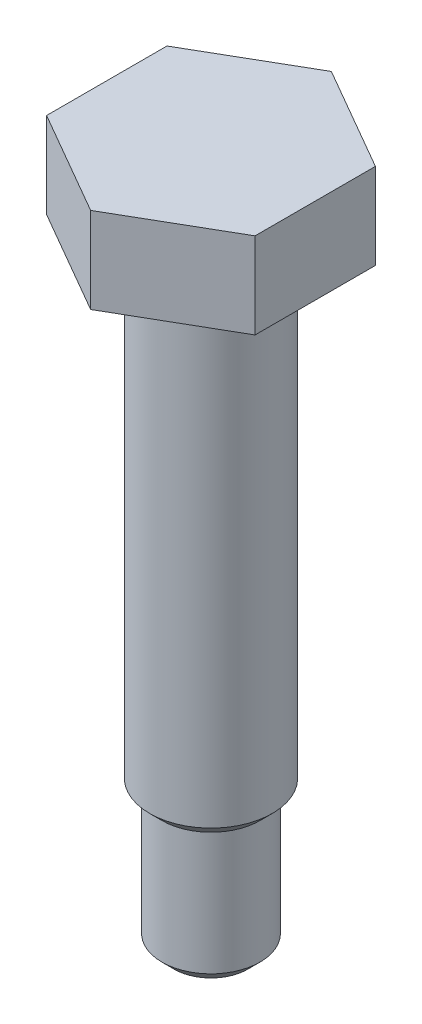
SolidWorks part; units mm, degrees
material "35"
ref_plane "前视基准面" through (0, 0, 0) normal (0, 0, 1) x (1, 0, 0)
ref_plane "上视基准面" through (0, 0, 0) normal (0, 1, 0) x (1, 0, 0)
ref_plane "右视基准面" through (0, 0, 0) normal (1, 0, 0) x (0, 0, -1)
sketch "草图1" plane through (0, 0, 0) normal (0, 1, 0) x (1, 0, 0)
  line L1 (0, 9.815) -> (-8.5, 4.9075)
  line L2 (-8.5, 4.9075) -> (-8.5, -4.9075)
  line L3 (-8.5, -4.9075) -> (0, -9.815)
  line L4 (0, -9.815) -> (8.5, -4.9075)
  line L5 (8.5, -4.9075) -> (8.5, 4.9075)
  line L6 (8.5, 4.9075) -> (0, 9.815)
  circle A0 centre (0, 0) radius 8.5 construction
  dimension "D1" = 17
extrude "凸台-拉伸1" add sketch "草图1" along normal blind 7
sketch "草图2" plane through (0, 0, 0) normal (0, 0, 1) x (1, 0, 0)
  line L0 (0, 0) -> (0, -50)
  line L1 (0, -50) -> (4, -50)
  line L2 (4, -50) -> (4, -39)
  line L3 (4, -39) -> (5, -38)
  line L4 (5, -38) -> (5, 0)
  line L5 (0, 0) -> (8.5, 0) construction
  line L6 (5, 0) -> (0, 0)
  dimension "D1" = 50
  dimension "D2" = 4
  dimension "D3" = 38
  dimension "D4" = 5
  dimension "D5" = 1
revolve "旋转1" add sketch "草图2" angle 360 about L0
cosmetic thread "装饰螺纹线1" parameters "D2"=6.647
chamfer "倒角1" distance 1 angle 45 1 edges at (0, -50, 4)
fillet "圆角1" radius 0.5 1 edges at (0, 0, 5)
